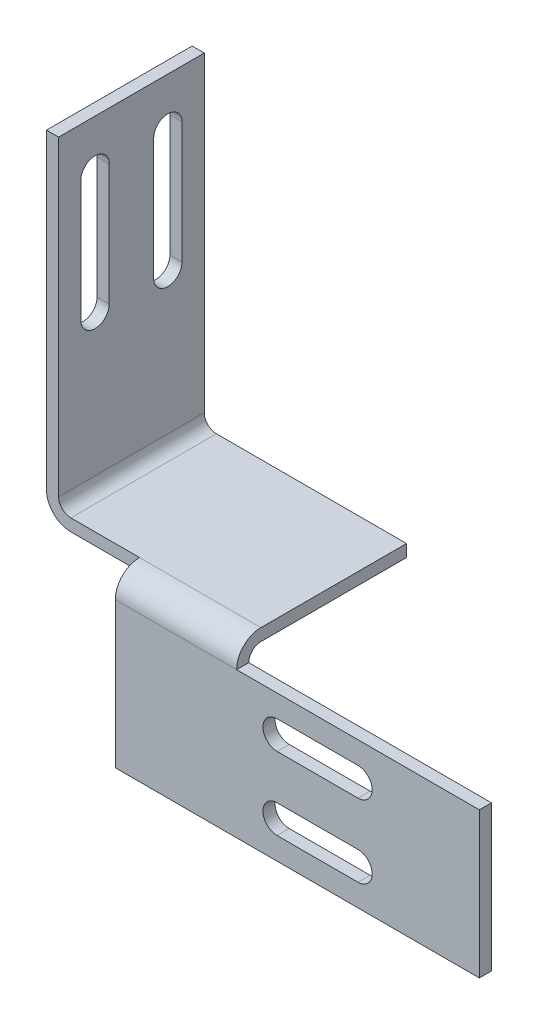
from build123d import *

# Parameters (mm, degrees)
EXTRUDE_THIN1_DEPTH      = 18
FILLET2_R                = 1.5
FILLET3_R                = 3
BOSS_EXTRUDE1_DEPTH      = 30
BOSS_EXTRUDE1_DEPTH_BACK = 15
SKETCH5_W                = 3
SKETCH5_H                = 3
CUT_EXTRUDE2_DEPTH       = 30
CUT_EXTRUDE3_DEPTH       = 73.341205409
CUT_EXTRUDE4_DEPTH       = 10


with BuildPart() as part:
    # Sketch1 → Extrude-Thin1 (new body)
    with BuildSketch(Plane.XY):
        Polygon((25, 0), (0, 0), (0, 40), (-1.5, 40), (-1.5, -1.5), (25, -1.5), align=None)
    extrude(amount=EXTRUDE_THIN1_DEPTH)

    # Fillet2
    fillet2_edges = [part.edges().sort_by_distance(p)[0] for p in [
        (0, 0, 9),
    ]]
    fillet(fillet2_edges, radius=FILLET2_R)

    # Fillet3
    fillet3_edges = [part.edges().sort_by_distance(p)[0] for p in [
        (-1.5, -1.5, 9),
    ]]
    fillet(fillet3_edges, radius=FILLET3_R)

    # Sketch4 → Boss-Extrude1 (add, two sides: drawn at the far end of the back side and taken through both)
    with BuildSketch(Plane(origin=(25, 0, 0), x_dir=(0, 0, -1), z_dir=(1, 0, 0)).offset(-BOSS_EXTRUDE1_DEPTH_BACK)):
        with BuildLine():
            Line((-21, -3), (-21, -21))
            Line((-21, -21), (-19.5, -21))
            Line((-19.5, -21), (-19.5, -3))
            ThreePointArc((-19.5, -3), (-19.060660172, -1.939339828), (-18, -1.5))
            Line((-18, -1.5), (-18, 0))
            ThreePointArc((-18, 0), (-20.121320344, -0.878679656), (-21, -3))
        make_face()
    extrude(amount=BOSS_EXTRUDE1_DEPTH + BOSS_EXTRUDE1_DEPTH_BACK)

    # Sketch5 → Cut-Extrude2 (cut)
    with BuildSketch(Plane(origin=(55, 0, 0), x_dir=(0, 0, -1), z_dir=(1, 0, 0))):
        with Locations((-19.5, -1.5)):
            Rectangle(SKETCH5_W, SKETCH5_H)
    extrude(amount=-CUT_EXTRUDE2_DEPTH, mode=Mode.SUBTRACT)

    # Sketch6 → Cut-Extrude3 (cut, through all)
    with BuildSketch(Plane.ZY.offset(1.5)):
        with BuildLine():
            Line((6.25, 34), (6.25, 19))
            ThreePointArc((6.25, 19), (4.5, 17.25), (2.75, 19))
            Line((2.75, 19), (2.75, 34))
            ThreePointArc((2.75, 34), (4.5, 35.75), (6.25, 34))
        make_face()
        with BuildLine():
            Line((11.75, 34), (11.75, 19))
            ThreePointArc((11.75, 19), (13.5, 17.25), (15.25, 19))
            Line((15.25, 19), (15.25, 34))
            ThreePointArc((15.25, 34), (13.5, 35.75), (11.75, 34))
        make_face()
    extrude(amount=-CUT_EXTRUDE3_DEPTH, mode=Mode.SUBTRACT)

    # Sketch7 → Cut-Extrude4 (cut)
    with BuildSketch(Plane.XY.offset(21)):
        with BuildLine():
            Line((30, -5.75), (40, -5.75))
            ThreePointArc((40, -5.75), (41.75, -7.5), (40, -9.25))
            Line((40, -9.25), (30, -9.25))
            ThreePointArc((30, -9.25), (28.25, -7.5), (30, -5.75))
        make_face()
        with BuildLine():
            Line((30, -18.25), (40, -18.25))
            ThreePointArc((40, -18.25), (41.75, -16.5), (40, -14.75))
            Line((40, -14.75), (30, -14.75))
            ThreePointArc((30, -14.75), (28.25, -16.5), (30, -18.25))
        make_face()
    extrude(amount=-CUT_EXTRUDE4_DEPTH, mode=Mode.SUBTRACT)


solid = part.part
